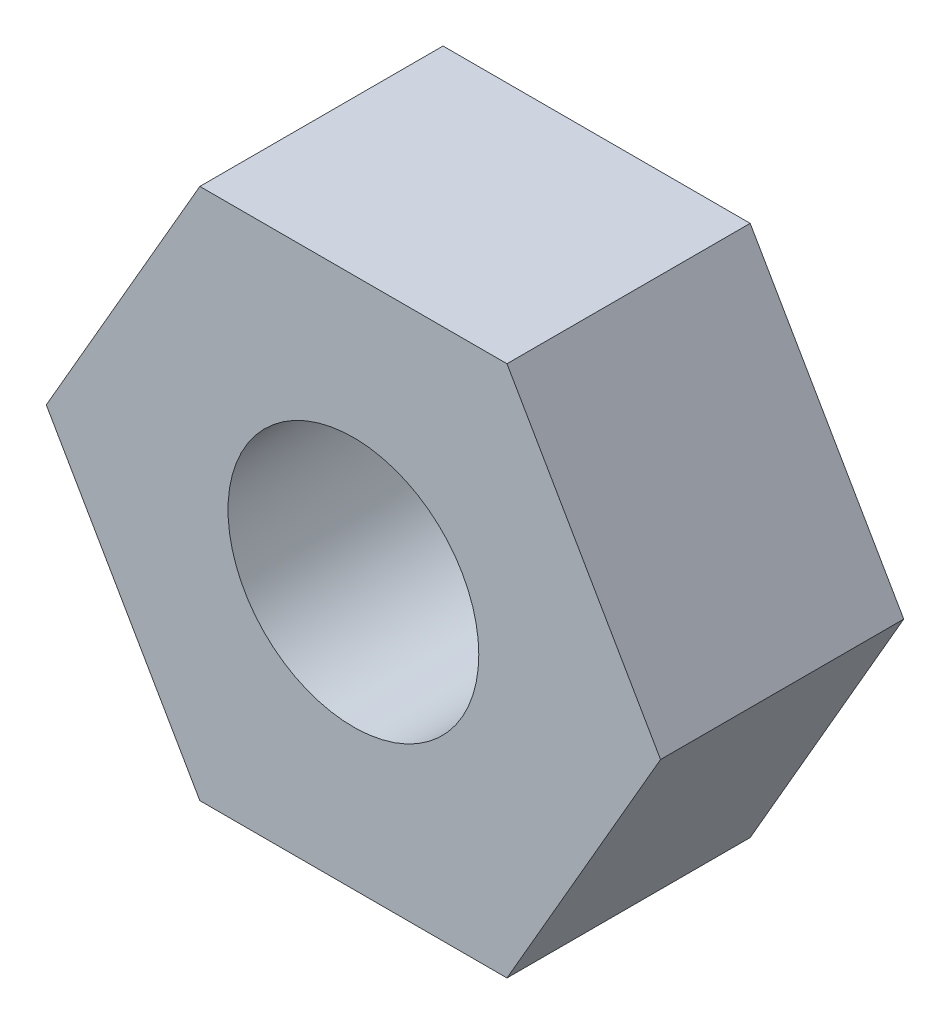
from build123d import *

# Parameters (mm, degrees)
SKETCH_1_R      = 1.65
EXTRUDE_1_DEPTH = 1.6


with BuildPart() as part:
    # 草图1 → 凸台-拉伸1 (new, symmetric)
    with BuildSketch(Plane.XY):
        Polygon((4.041451884, 0), (2.020725942, 3.5), (-2.020725942, 3.5), (-4.041451884, 0), (-2.020725942, -3.5), (2.020725942, -3.5), align=None)
        Circle(SKETCH_1_R, mode=Mode.SUBTRACT)
    extrude(amount=EXTRUDE_1_DEPTH, both=True)


solid = part.part
